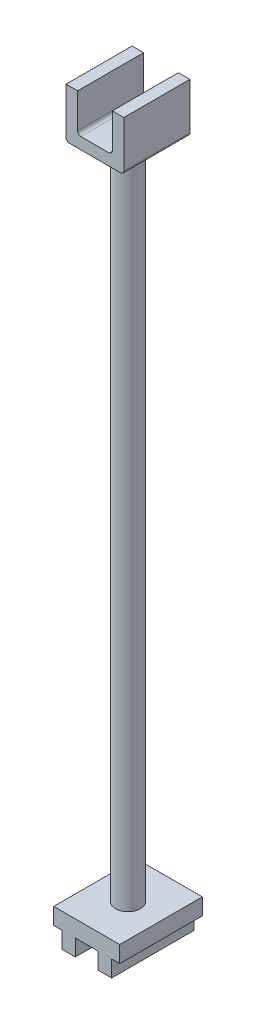
from build123d import *

# Parameters (mm, degrees)
BOSS_EXTRUDE1_DEPTH = 20
FILLET1_R           = 2
SKETCH2_R           = 7.5
BOSS_EXTRUDE2_DEPTH = 400
SKETCH3_W           = 40
SKETCH3_H           = 50
BOSS_EXTRUDE3_DEPTH = 10
SKETCH4_W           = 8.2
SKETCH4_H           = 50
BOSS_EXTRUDE4_DEPTH = 10


with BuildPart() as part:
    # Sketch1 → Boss-Extrude1 (new, symmetric)
    with BuildSketch(Plane.XY):
        Polygon((-10.5, 8), (-10.5, -8), (10.5, -8), (10.5, 8), (10.5, 15), (17.5, 15), (17.5, -15), (-17.5, -15), (-17.5, 15), (-10.5, 15), align=None)
    extrude(amount=BOSS_EXTRUDE1_DEPTH, both=True)

    # Fillet1
    fillet1_edges = [part.edges().sort_by_distance(p)[0] for p in [
        (17.5, -15, 0),
        (-17.5, -15, 0),
        (-10.5, -8, 0),
        (10.5, -8, 0),
    ]]
    fillet(fillet1_edges, radius=FILLET1_R)

    # Sketch2 → Boss-Extrude2 (add)
    with BuildSketch(Plane.XZ.offset(15)):
        with Locations(Location((0, 0, 0), (0, 0, 180))):
            Circle(SKETCH2_R)
    extrude(amount=BOSS_EXTRUDE2_DEPTH)

    # Sketch3 → Boss-Extrude3 (add)
    with BuildSketch(Plane.XZ.offset(415)):
        Rectangle(SKETCH3_W, SKETCH3_H)
    extrude(amount=BOSS_EXTRUDE3_DEPTH)

    # Sketch4 → Boss-Extrude4 (add)
    with BuildSketch(Plane.XZ.offset(425)):
        with Locations((-11, 0)):
            Rectangle(SKETCH4_W, SKETCH4_H)
        with Locations((11, 0)):
            Rectangle(SKETCH4_W, SKETCH4_H)
    extrude(amount=BOSS_EXTRUDE4_DEPTH)


solid = part.part
